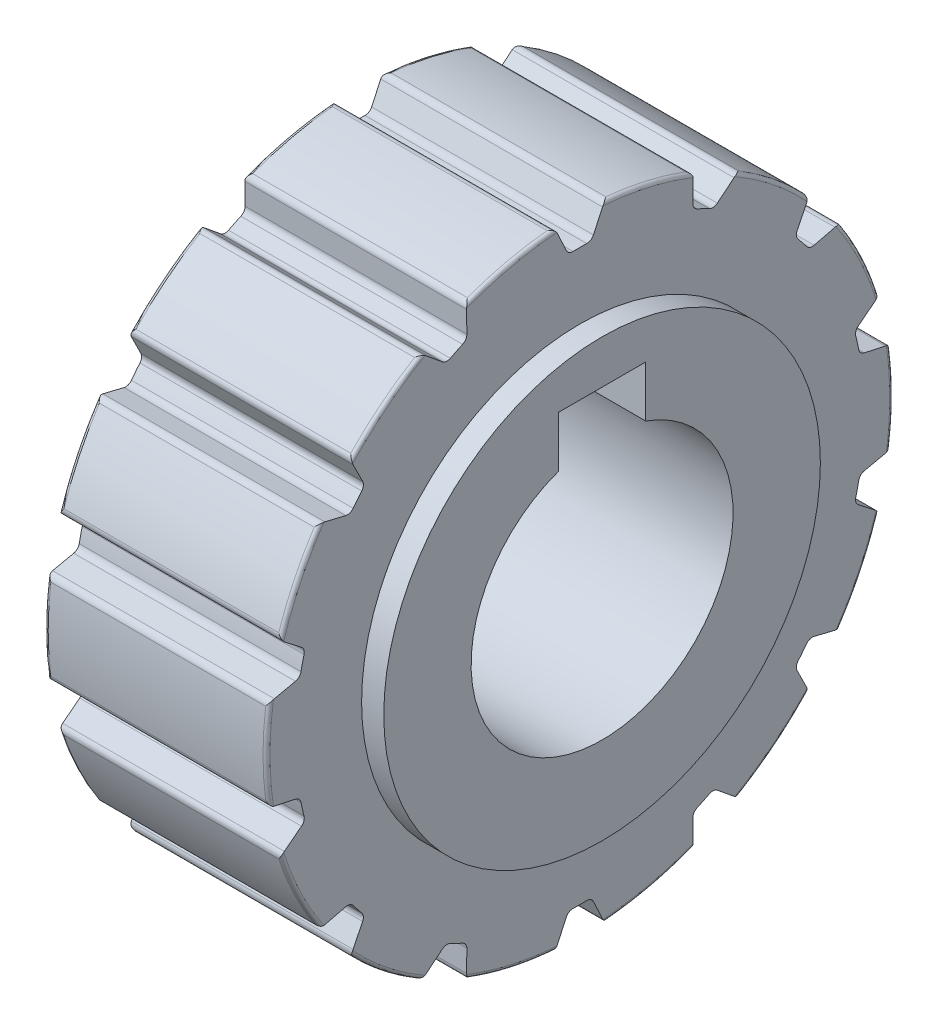
from build123d import *

# Parameters (mm, degrees)
CHAMFER1_SIZE       = 1
SKETCH4_W           = 2
SKETCH4_H           = 1.1421205637235645
CUT_EXTRUDE1_DEPTH  = 30.603638891008007
FILLET1_R           = 2
CUT_EXTRUDE3_REACH  = 30.97
CIRPATTERN3_COUNT   = 14
SKETCH7_R           = 15
BOSS_EXTRUDE1_DEPTH = 12.7
BOSS_EXTRUDE2_START = -15.24
SKETCH8_R           = 12.5
BOSS_EXTRUDE2_DEPTH = 15.24
CUT_EXTRUDE4_DEPTH  = 30.55708472681763


with BuildPart() as part:
    # Sketch1 → Revolve1 (revolve)
    with BuildSketch(Plane.XY, mode=Mode.PRIVATE) as revolve1_sk:
        with BuildLine():
            Line((-1.2699999999999934, 3.5891999999999866), (-1.2700000000000071, 7.178400000000002))
            Line((-1.2700000000000071, 7.178400000000002), (4.063999999999977, 7.391703116710807))
            Line((4.063999999999977, 7.391703116710807), (4.063999999999977, 14.194283339648894))
            Line((4.063999999999977, 14.194283339648894), (0, 14.356800000000003))
            Line((0, 14.356800000000003), (0, 17.745999999999984))
            ThreePointArc((0, 17.745999999999984), (0.05857864376269051, 17.887421356237294), (0.20000000000000004, 17.94600000000002))
            Line((0.20000000000000004, 17.94600000000002), (12.499999999999996, 17.94600000000002))
            ThreePointArc((12.499999999999996, 17.94600000000002), (12.641421356237311, 17.887421356237297), (12.700000000000003, 17.745999999999984))
            Line((12.700000000000003, 17.745999999999984), (12.700000000000003, 14.356800000000003))
            Line((12.700000000000003, 14.356800000000003), (8.636000000000019, 14.194283339648894))
            Line((8.636000000000019, 14.194283339648894), (8.636000000000019, 7.3917031167108345))
            Line((8.636000000000019, 7.3917031167108345), (13.97000000000001, 7.178400000000002))
            Line((13.97000000000001, 7.178400000000002), (13.969999999999997, 3.5891999999999866))
            Line((13.969999999999997, 3.5891999999999866), (-1.2699999999999934, 3.5891999999999866))
        make_face()
    revolve(revolve1_sk.sketch.rotate(Axis((0, 0, 0), (1, 0, 0)), 90), axis=Axis((0, 0, 0), (1, 0, 0)))

    # Chamfer1
    chamfer1_edges = [part.edges().sort_by_distance(p)[0] for p in [
        (-1.2699999999999934, -8.4e-16, -3.5891999999999866),
        (13.969999999999997, -8.4e-16, -3.5891999999999866),
    ]]
    chamfer(chamfer1_edges, length=CHAMFER1_SIZE)

    # Sketch4 → Cut-Extrude1 (cut, through all)
    with BuildSketch(Plane.ZY.offset(1.2700000000000002)):
        with Locations((0, 4.01813971813822)):
            Rectangle(SKETCH4_W, SKETCH4_H)
    extrude(amount=-CUT_EXTRUDE1_DEPTH, mode=Mode.SUBTRACT)

    # Fillet1
    fillet1_edges = [part.edges().sort_by_distance(p)[0] for p in [
        (8.636000000000019, -1.73e-15, -7.3917031167108345),
        (8.636000000000019, -3.31e-15, -14.194283339648894),
        (4.063999999999977, -3.31e-15, -14.194283339648894),
        (4.063999999999977, -1.73e-15, -7.391703116710807),
    ]]
    fillet(fillet1_edges, radius=FILLET1_R)

    # Sketch6 → Cut-Extrude3 (cut, up to next)
    with BuildSketch(Plane(origin=(0, 0, 0), x_dir=(0, 0, -1), z_dir=(1, 0, 0)), mode=Mode.PRIVATE) as cut_extrude3_sk1:
        with BuildLine():
            Line((-1.2974731850063128, 17.649694928596926), (-0.7743578697036396, 16.527870514705807))
            ThreePointArc((-0.7743578697036396, 16.527870514705807), (-0.6188798034969856, 16.35272288086002), (-0.3928868220217499, 16.291263178313756))
            ThreePointArc((-0.3928868220217499, 16.291263178313756), (1.185e-14, 16.295999999999996), (0.3928868220217721, 16.291263178313752))
            ThreePointArc((0.3928868220217721, 16.291263178313752), (0.6188798034970011, 16.35272288086005), (0.7743578697036666, 16.527870514705832))
            Line((0.7743578697036666, 16.527870514705832), (1.2974731850063508, 17.649694928596972))
            ThreePointArc((1.2974731850063508, 17.649694928596972), (1.4529141154090697, 17.818790175869665), (1.6773882275796792, 17.867436434306327))
            ThreePointArc((1.6773882275796792, 17.867436434306327), (1.8664624372237058, 17.848675972475746), (2.0553274268185486, 17.827914773426766))
            Line((2.0553274268185486, 17.827914773426766), (17.48728008472912, 50.92184404529182))
            ThreePointArc((17.48728008472912, 50.92184404529182), (2.721e-14, 53.840868916974074), (-17.48728008472908, 50.92184404529183))
            Line((-17.48728008472908, 50.92184404529183), (-2.0553274268185087, 17.82791477342675))
            ThreePointArc((-2.0553274268185087, 17.82791477342675), (-1.8664624372236707, 17.84867597247574), (-1.6773882275796381, 17.86743643430632))
            ThreePointArc((-1.6773882275796381, 17.86743643430632), (-1.4529141154090195, 17.818790175869655), (-1.2974731850063128, 17.649694928596926))
        make_face()
    cut_extrude3_tool1 = extrude(cut_extrude3_sk1.sketch, amount=CUT_EXTRUDE3_REACH, mode=Mode.PRIVATE) & part.part
    cut_extrude3 = cut_extrude3_tool1.solids().sort_by_distance((0, 39.910455, 0))[0]
    add(cut_extrude3, mode=Mode.SUBTRACT)

    # CirPattern3: Cut-Extrude3 ×14 about axis
    cirpattern3_axis = Axis((0, -1e-17, -5e-17), (1, 0, 0))
    for i in range(1, CIRPATTERN3_COUNT):
        add(cut_extrude3.rotate(cirpattern3_axis, i * 360 / CIRPATTERN3_COUNT), mode=Mode.SUBTRACT)

    # Sketch7 → Boss-Extrude1 (add)
    with BuildSketch(Plane.ZY):
        Circle(SKETCH7_R)
    extrude(amount=-BOSS_EXTRUDE1_DEPTH)

    # Sketch8 → Boss-Extrude2 (add)
    with BuildSketch(Plane(origin=(13.970000000000002, 0, 0), x_dir=(0, 0, -1), z_dir=(1, 0, 0)).offset(BOSS_EXTRUDE2_START)):
        Circle(SKETCH8_R)
    extrude(amount=BOSS_EXTRUDE2_DEPTH)

    # Sketch9 → Cut-Extrude4 (cut, through all)
    with BuildSketch(Plane.ZY.offset(1.2700000000000002)):
        with BuildLine():
            Line((-2.5, 7.0710678118654755), (-2.5, 10))
            Line((-2.5, 10), (2.5, 10))
            Line((2.5, 10), (2.5, 7.0710678118654755))
            ThreePointArc((2.5, 7.0710678118654755), (-1.38e-15, -7.5), (-2.5, 7.0710678118654755))
        make_face()
    extrude(amount=-CUT_EXTRUDE4_DEPTH, mode=Mode.SUBTRACT)


solid = part.part
